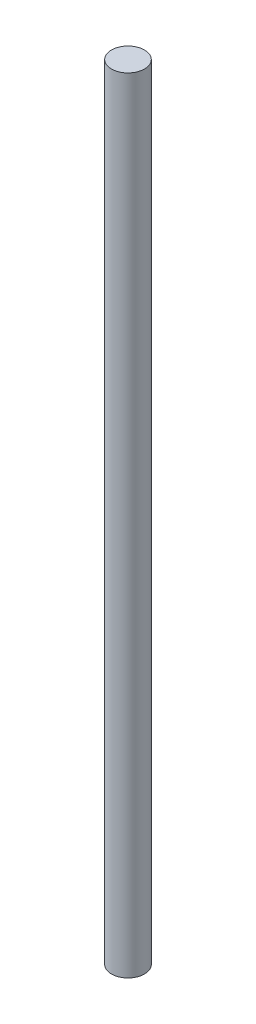
SolidWorks part; units mm, degrees
material "普通碳钢"
ref_plane "Front Plane" through (0, 0, 0) normal (0, 0, 1) x (1, 0, 0)
ref_plane "Top Plane" through (0, 0, 0) normal (0, 1, 0) x (1, 0, 0)
ref_plane "Right Plane" through (0, 0, 0) normal (1, 0, 0) x (0, 0, -1)
sketch "Sketch1" plane through (0, 0, 0) normal (0, 1, 0) x (1, 0, 0)
  circle A0 centre (0, 0) radius 8
  dimension "D1" = 16
extrude "Boss-Extrude1" add sketch "Sketch1" along normal blind 380
cosmetic thread "Cosmetic Thread1" parameters "D2"=13.835
sketch "Sketch2" plane through (0, 0, 0) normal (0, 0, 1) x (1, 0, 0)
  line L0 (0, 340) -> (0, 100) construction
  line L1 (3, 340) -> (3, 100)
  line L2 (-3, 340) -> (-3, 100)
  line L3 (8, 380) -> (-8, 380) construction
  arc A0 (3, 340) -> (-3, 340) centre (0, 340) ccw
  arc A1 (-3, 100) -> (3, 100) centre (0, 100) ccw
  point P3 (0, 220)
  dimension "D2" = 40
  dimension "D1" = 6
  dimension "D3" = 240
